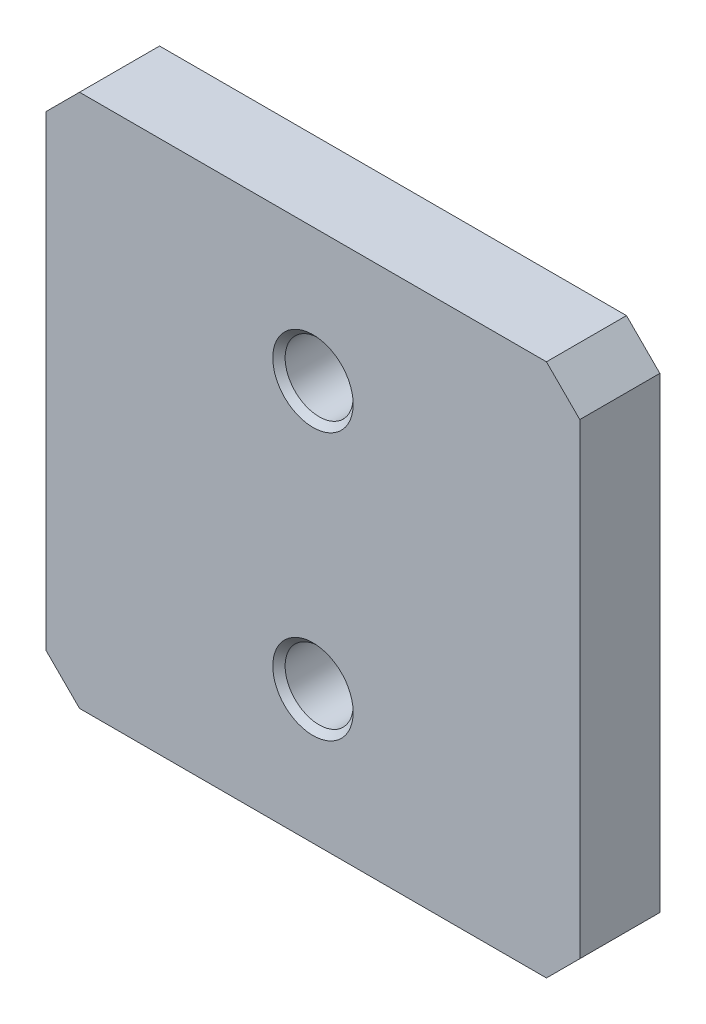
from build123d import *

# Parameters (mm, degrees)
SKETCH_1_W                    = 80
SKETCH_1_H                    = 80
EXTRUDE_1_DEPTH               = 12
CHAMFER_1_SIZE                = 5
HOLE_WIZARD_M12_1_D           = 10.2
HOLE_WIZARD_M12_1_DEPTH       = 32.75
HOLE_WIZARD_M12_1_CSINK_D     = 12.05
HOLE_WIZARD_M12_1_CSINK_ANGLE = 90
HOLE_WIZARD_M12_1_TIP         = 3.064389157


with BuildPart() as part:
    # 草图1 → 凸台-拉伸1 (new body)
    with BuildSketch(Plane.XY):
        Rectangle(SKETCH_1_W, SKETCH_1_H)
    extrude(amount=EXTRUDE_1_DEPTH)

    # 倒角1
    chamfer_1_edges = [part.edges().sort_by_distance(p)[0] for p in [
        (40, -40, 6),
        (-40, -40, 6),
        (-40, 40, 6),
        (40, 40, 6),
    ]]
    chamfer(chamfer_1_edges, length=CHAMFER_1_SIZE)

    # M12 螺纹孔1
    with Locations(Plane(origin=(0, 20, 12), x_dir=(1, 0, 0), z_dir=(0, 0, 1))):
        with Locations((0, 0), (0, -40)):
            CounterSinkHole(HOLE_WIZARD_M12_1_D / 2, HOLE_WIZARD_M12_1_CSINK_D / 2, depth=HOLE_WIZARD_M12_1_DEPTH, counter_sink_angle=HOLE_WIZARD_M12_1_CSINK_ANGLE)
            with Locations((0, 0, -(HOLE_WIZARD_M12_1_DEPTH + HOLE_WIZARD_M12_1_TIP / 2))):  # 118° drill point
                Cone(0, HOLE_WIZARD_M12_1_D / 2, HOLE_WIZARD_M12_1_TIP, mode=Mode.SUBTRACT)


solid = part.part
